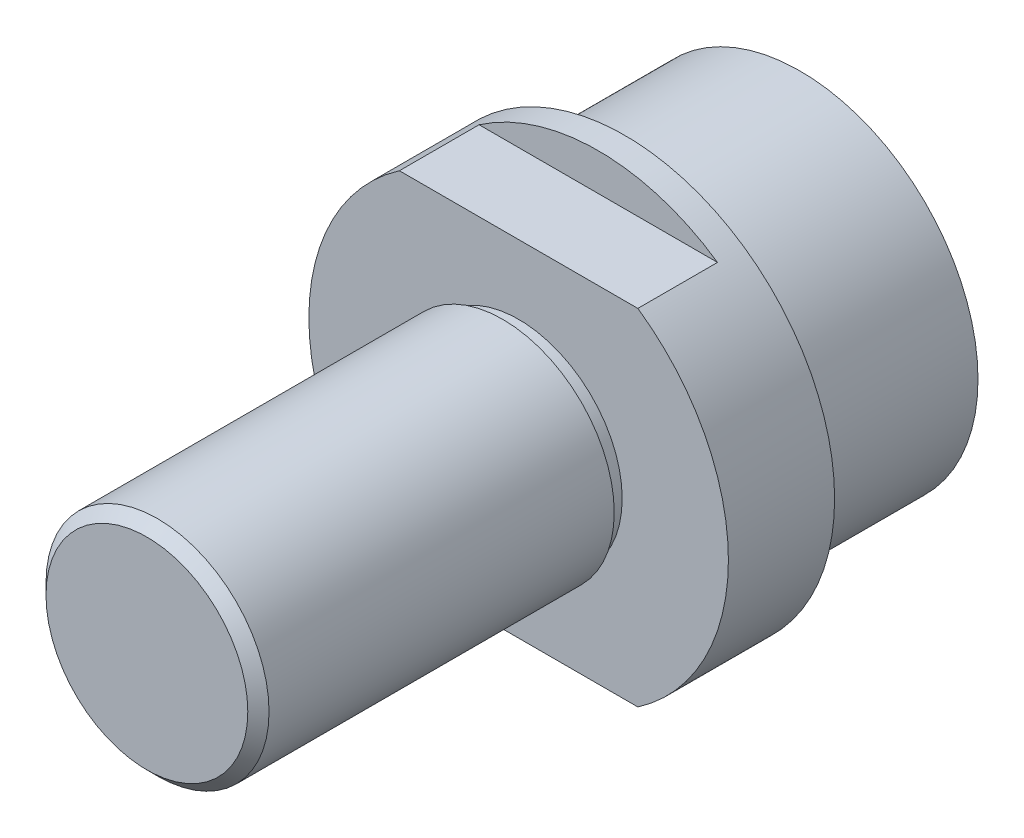
SolidWorks part; units mm, degrees
ref_plane "Front Plane" through (0, 0, 0) normal (0, 0, 1) x (1, 0, 0)
ref_plane "Top Plane" through (0, 0, 0) normal (0, 1, 0) x (1, 0, 0)
ref_plane "Right Plane" through (0, 0, 0) normal (1, 0, 0) x (0, 0, -1)
sketch "Sketch1" plane through (0, 0, 0) normal (0, 0, 1) x (1, 0, 0)
  circle A0 centre (0, 0) radius 33.5
  dimension "D1" = 67
extrude "Boss-Extrude1" add sketch "Sketch1" along normal blind 33
sketch "Sketch2" plane through (0, 0, 33) normal (0, 0, 1) x (1, 0, 0)
  circle A0 centre (0, 0) radius 39.5
  dimension "D1" = 79
extrude "Boss-Extrude2" add sketch "Sketch2" along normal blind 20 contours A0
sketch "Sketch3" plane through (0, 0, 53) normal (0, 0, 1) x (1, 0, 0)
  line L0 (-22.4499, 32.5) -> (22.4499, 32.5)
  line L1 (-22.4499, -32.5) -> (22.4499, -32.5)
  circle A0 centre (0, 0) radius 39.5 construction
  arc A1 (-22.4499, -32.5) -> (22.4499, -32.5) centre (0, 0) ccw
  arc A2 (22.4499, 32.5) -> (-22.4499, 32.5) centre (0, 0) ccw
  dimension "D1" = 65
  dimension "D2" = 32.5
extrude "Cut-Extrude1" cut sketch "Sketch3" against normal blind 15
sketch "Sketch4" plane through (0, 0, 53) normal (0, 0, 1) x (1, 0, 0)
  circle A0 centre (0, 0) radius 19.5
  dimension "D1" = 39
extrude "Boss-Extrude3" add sketch "Sketch4" along normal blind 3
sketch "Sketch5" plane through (0, 0, 56) normal (0, 0, 1) x (1, 0, 0)
  circle A0 centre (0, 0) radius 21
  dimension "D1" = 42
extrude "Boss-Extrude4" add sketch "Sketch5" along normal blind 67
chamfer "Chamfer1" distance 2 angle 45 1 edges at (21, 0, 123)
